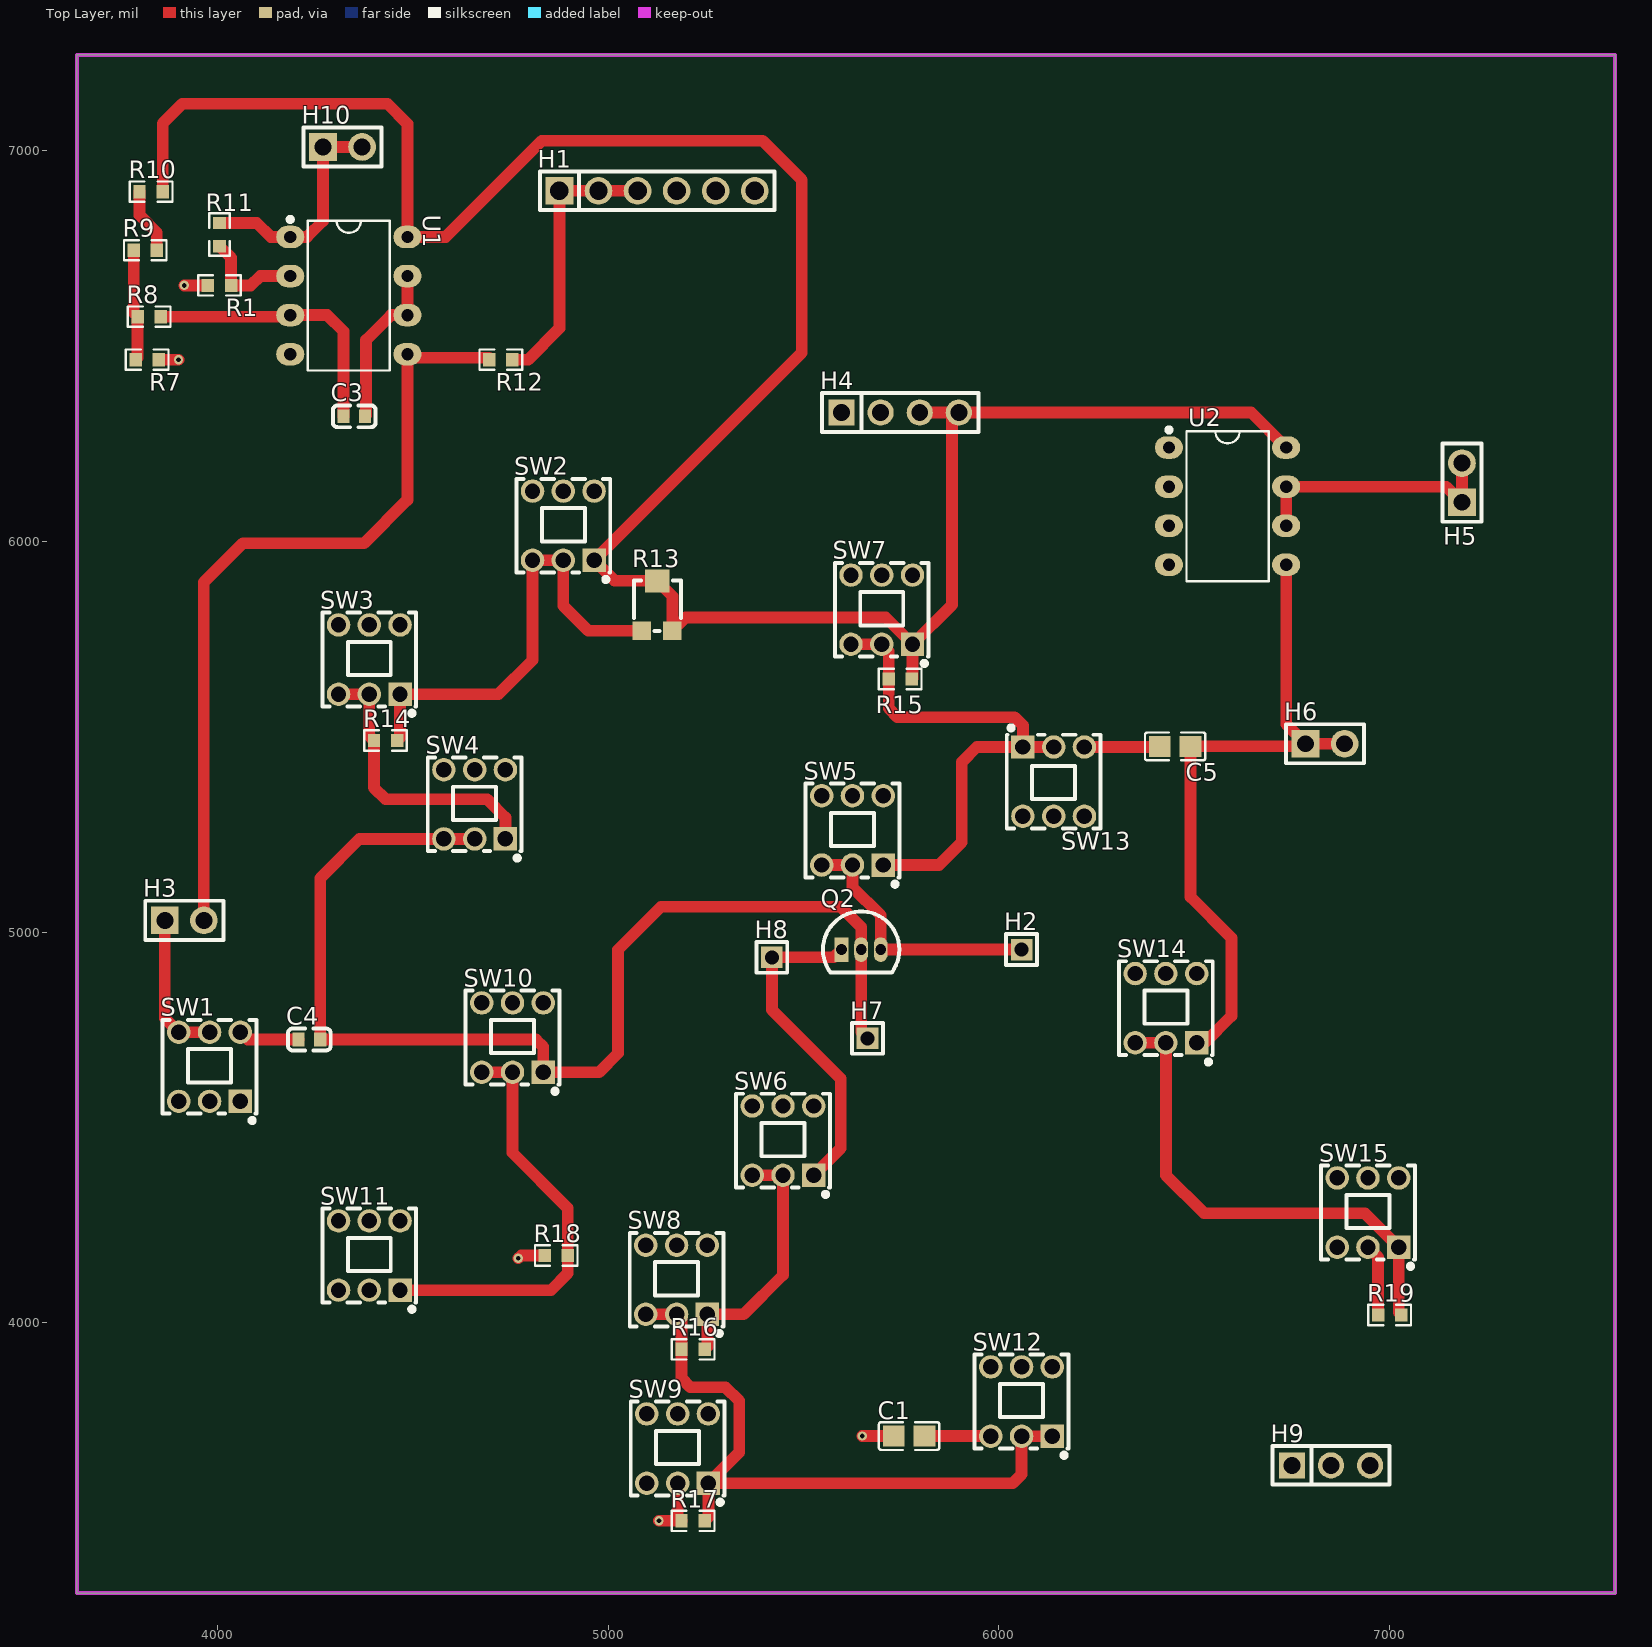
[diagram p0: Top Layer view]
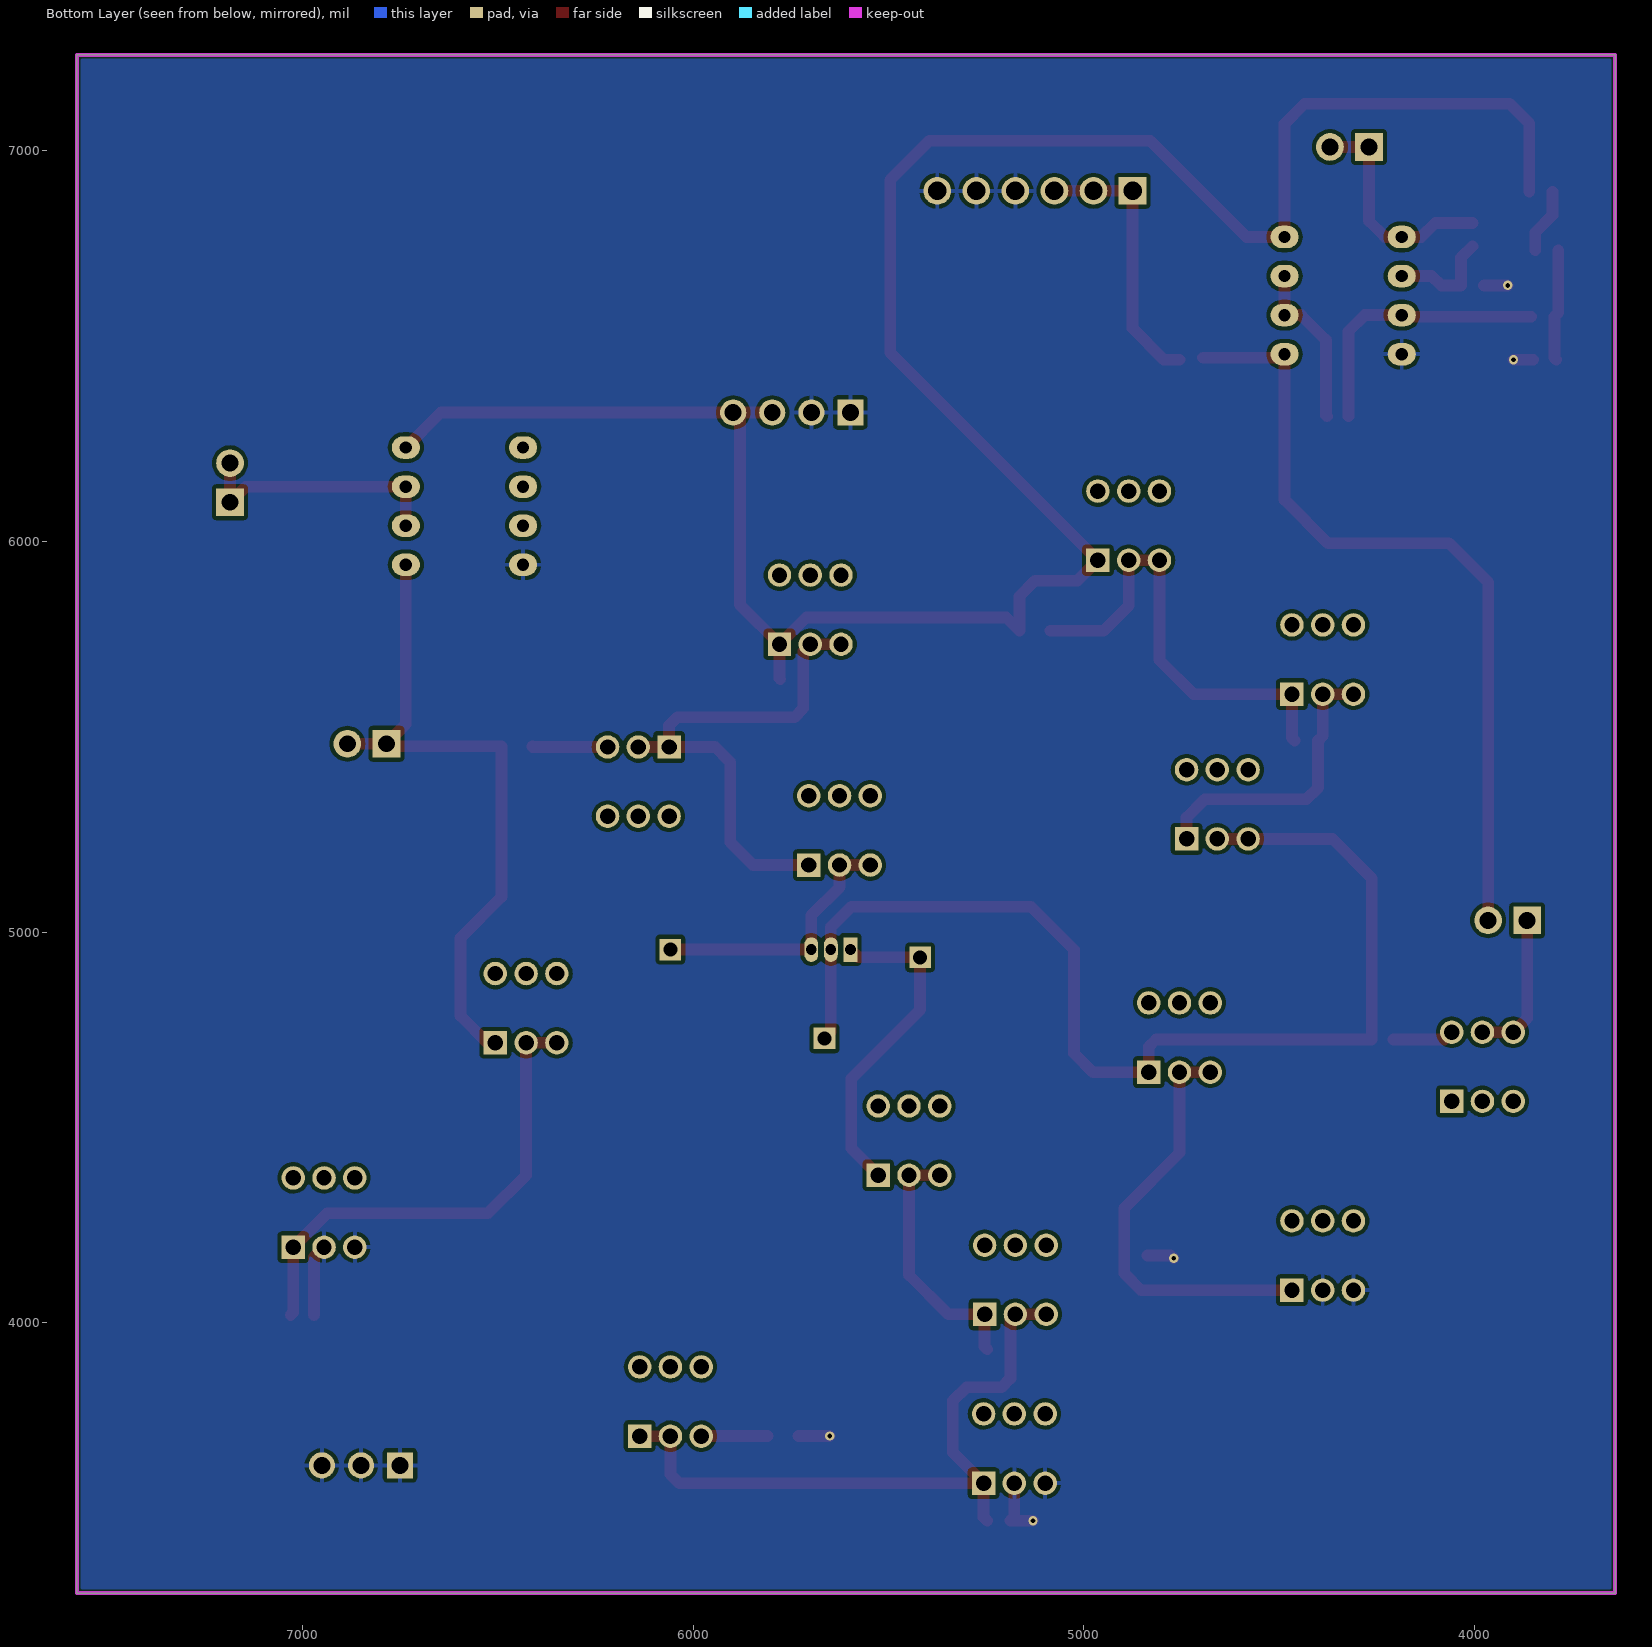
[diagram p1: Bottom Layer view, seen from below]
# Altium PCB MISC52134.pcbdoc
Units mil, origin at the board's own origin, x right, y up, seen from the top; angles counter-clockwise.
Board outline 3937.01 x 3937.01 mil, 2 copper layers (Top Layer, Bottom Layer), stack 62.206 mil thick; 46 components, 26 nets, 170 pads, 5 vias.

## Layer stack, top to bottom
Top Solder Mask Layer: solder mask 0.394, Dk 3.3
Top Layer: signal copper 1.379
Dielectric1: surface 59.449, FR4, Dk 4.5
Bottom Layer: signal copper 1.378
Bottom Solder Mask Layer: solder mask 0.394, Dk 3.3

## Board outline
3640,7245 3640,3307.99 7577.01,3307.99 7577.01,7245

## Design rules (kind name [scope] priority, off if disabled: settings)
BoardOutlineClearance copperThickness2oz_1 [All] p2 off: genericclearance=7.99 ignorepadtopadclearanceinfootprint=FALSE except(0: Arc-SplitContinuation Track-SplitContinuation SMDPad-SplitContinuation THPad-SplitContinuation Via-SplitContinuation Fill-SplitContinuation Region-SplitContinuation Poly-SplitContinuation Text-SplitContinuation Hole-SplitContinuation; 5.98: Arc-CutoutEdge SMDPad-CutoutEdge THPad-CutoutEdge Via-CutoutEdge Fill-CutoutEdge Region-CutoutEdge Text-CutoutEdge; 6.93: Hole-OutlineEdge Hole-CutoutEdge; 10: Poly-OutlineEdge Poly-CutoutEdge; 11.81: Arc-OutlineEdge Track-OutlineEdge SMDPad-OutlineEdge THPad-OutlineEdge Via-OutlineEdge Fill-OutlineEdge Region-OutlineEdge Text-OutlineEdge Track-CutoutEdge)
BoardOutlineClearance copperThickness1oz_1 [All] p4: genericclearance=4.02 ignorepadtopadclearanceinfootprint=FALSE except(0: Arc-SplitContinuation Track-SplitContinuation SMDPad-SplitContinuation THPad-SplitContinuation Via-SplitContinuation Fill-SplitContinuation Region-SplitContinuation Poly-SplitContinuation Text-SplitContinuation Hole-SplitContinuation; 6: SMDPad-CutoutEdge THPad-CutoutEdge Via-CutoutEdge Fill-CutoutEdge Region-CutoutEdge Text-CutoutEdge; 6.93: Hole-OutlineEdge Hole-CutoutEdge; 10: Poly-OutlineEdge Poly-CutoutEdge; 11.8: Arc-OutlineEdge Track-OutlineEdge SMDPad-OutlineEdge THPad-OutlineEdge Via-OutlineEdge Fill-OutlineEdge Region-OutlineEdge Text-OutlineEdge; 11.81: Arc-CutoutEdge Track-CutoutEdge)
Clearance copperThickness2oz [All] p1 off: gap=7.99 ignorepadtopadclearanceinfootprint=FALSE except(5.98: SMDPad-Track SMDPad-SMDPad THPad-Track SMDPad-THPad THPad-THPad Track-Via SMDPad-Via THPad-Via Via-Via Fill-Track Region-Track Fill-SMDPad Region-SMDPad Fill-THPad Region-THPad Fill-Via Region-Via Fill-Fill Fill-Region Region-Region Arc-Track Arc-SMDPad Arc-THPad Arc-Via Fill-Arc Region-Arc Arc-Arc Text-Track SMDPad-Text Text-THPad Text-Via Fill-Text Region-Text Arc-Text Text-Text; 6.93: Hole-Track Hole-SMDPad Hole-THPad Hole-Via Fill-Hole Region-Hole Hole-Arc Hole-Text; 10: Poly-Track Poly-SMDPad Poly-THPad Poly-Via Poly-Fill Poly-Region Poly-Poly Poly-Arc Poly-Text Poly-Hole)
Clearance copperThickness1oz [All] p3: gap=4.02 ignorepadtopadclearanceinfootprint=FALSE except(5.98: SMDPad-Track SMDPad-SMDPad THPad-Track SMDPad-THPad THPad-THPad Track-Via SMDPad-Via THPad-Via Via-Via Fill-Track Region-Track Fill-SMDPad Region-SMDPad Fill-THPad Region-THPad Fill-Via Region-Via Fill-Fill Fill-Region Region-Region; 6: Arc-Track Arc-SMDPad Arc-THPad Arc-Via Fill-Arc Region-Arc Arc-Arc Text-Track SMDPad-Text Text-THPad Text-Via Fill-Text Region-Text Arc-Text Text-Text; 6.93: Hole-Track Hole-SMDPad Hole-THPad Hole-Via Fill-Hole Region-Hole Hole-Arc Hole-Text; 10: Poly-Track Poly-SMDPad Poly-THPad Poly-Via Poly-Fill Poly-Region Poly-Poly Poly-Arc Poly-Text Poly-Hole)
Creepage creepage [All] p1: checkdistance=0 ignoreinternallayers=TRUE applytopolygonpour=TRUE
DiffPairsRouting differentialPair [All] p1: maxlimit=6 minlimit=6 mostfreqgap=6 toplayer_minwidth=5 toplayer_prefwidth=10 toplayer_maxwidth=100 toplayer_mingap=6 toplayer_prefgap=6 toplayer_maxgap=6 bottomlayer_minwidth=5 bottomlayer_prefwidth=10 bottomlayer_maxwidth=100 bottomlayer_mingap=6 bottomlayer_prefgap=6 bottomlayer_maxgap=6 maxuncoupledlength=10
HoleToHoleClearance otherClearance [All] p1: gap=11.81 allowstackedmicrovias=TRUE
Length netLength [All] p1: minlimit=0 maxlimit=0
MatchedLengths netLengthTolerance [All] p1: tolerance=1000
PasteMaskExpansion pasteMaskExpansion [All] p1: expansion=0
PlaneConnect innerPlane [All] p1: planeconnectstyle=Relief reliefexpansion=20 reliefentries=4 reliefconductorwidth=10 reliefairgap=10
PolygonConnect copperRegion [(InNet('GND'))] p1: connectstyle=Relief reliefconductorwidth=10 reliefentries=4 polygonreliefangle="90 Angle" airgapwidth=10 via.connectstyle=Relief via.reliefconductorwidth=10 via.reliefentries=4 via.polygonreliefangle="90 Angle" via.airgapwidth=10
RoutingVias viaSize [All] p1: holewidth=12.01 width=24.02 viastyle="Through Hole" minholewidth=11.81 minwidth=19.68 maxholewidth=248.03 maxwidth=393.7
SolderMaskExpansion solderMaskExpansion [IsVia] p1: expansion=-1000 istentingtop=TRUE
SolderMaskExpansion solderMaskExpansion [All] p2: expansion=2 istentingtop=FALSE
Width copperThickness2oz_2 [All] p1 off: maxlimit=100 minlimit=8 preferedwidth=10
Width copperThickness1oz_2 [All] p2: maxlimit=100 minlimit=5 preferedwidth=10

## Components (designator, comment, footprint, x,y, rotation, side; value= is the part's Value field where it differs from the comment)
C1 "100uF" C0805 5770,3710 r0 top
C3 "0.47uF" C0603 4350,6320 r0 top
C4 "10uF" C0603 4235,4725 r0 top
C5 "10uF" C0805 6450.98,5475.15 r180 top
H1 "" HDR-TH_6P-P2.54-V-M-1 5125,6897.06 r0 top
H2 "" HDR-TH_1P-V-M_XKB_X4611WV-01I-C28D40 6057.89,4955.13 r0 top
H3 "" HDR-TH_2P-P2.54-V-M-1 3915,5030 r0 top
H4 "" HDR-TH_4P-P2.54-V-M 5747.25,6329.7 r0 top
H5 "" HDR-TH_2P-P2.54-V-M-1 7185,6150 r90 top
H6 "" HDR-TH_2P-P2.54-V-M-1 6834.77,5481.89 r0 top
H7 "" HDR-TH_1P-V-M_XKB_X4611WV-01I-C28D40 5663.51,4727.83 r0 top
H8 "" HDR-TH_1P-V-M_XKB_X4611WV-01I-C28D40 5418.84,4935.13 r0 top
H9 "" HDR-TH_3P-P2.54-V-M 6850,3635 r0 top
H10 "" HDR-TH_2P-P2.54-V-M-1 4319.9,7009.39 r0 top
Q2 "2N2222A" TO-92-3_L4.9-W3.7-P1.27-L 5647.25,4955.13 r0 top
R1 "1kΩ" R0603 4005,6655 r180 top
R7 "1kΩ" R0603 3820,6465 r180 top
R8 "2kΩ" R0603 3825,6575 r0 top
R9 "100kΩ" R0603 3815,6745 r0 top
R10 "100kΩ" R0603 3830,6895 r0 top
R11 "20kΩ" R0603 4005,6785 r90 top
R12 "10KΩ" R0603 4725,6465 r180 top
R13 "100kΩ" RES-ADJ-SMD_JER33X-1-14 5125,5835 r0 top
R14 "39kΩ" R0603 4430,5490 r0 top
R15 "24kΩ" R0603 5747.25,5647.42 r0 top
R16 "100Ω" R0603 5217.25,3932.06 r0 top
R17 "1kΩ" R0603 5217.25,3493.05 r0 top
R18 "20KΩ" R0603 4866.92,4172.06 r0 top
R19 "2.4KΩ" R0603 7000,4020 r0 top
SW1 "5.8 ZSGT" SW-TH_5.8ZSGT 3979.58,4655.13 r0 top
SW2 "5.8 ZSGT" SW-TH_5.8ZSGT 4885,6040 r0 top
SW3 "5.8 ZSGT" SW-TH_5.8ZSGT 4388.4,5697.42 r0 top
SW4 "5.8 ZSGT" SW-TH_5.8ZSGT 4658.08,5326.89 r0 top
SW5 "5.8 ZSGT" SW-TH_5.8ZSGT 5625,5260 r0 top
SW6 "5.8 ZSGT" SW-TH_5.8ZSGT 5447.25,4466.08 r0 top
SW7 "5.8 ZSGT" SW-TH_5.8ZSGT 5700,5825 r0 top
SW8 "5.8 ZSGT" SW-TH_5.8ZSGT 5175,4110 r0 top
SW9 "5.8 ZSGT" SW-TH_5.8ZSGT 5177.56,3678.05 r0 top
SW10 "5.8 ZSGT" SW-TH_5.8ZSGT 4755,4730 r0 top
SW11 "5.8 ZSGT" SW-TH_5.8ZSGT 4388.4,4172.06 r0 top
SW12 "5.8 ZSGT" SW-TH_5.8ZSGT 6057.89,3798.37 r0 top
SW13 "5.8 ZSGT" SW-TH_5.8ZSGT 6140,5385 r180 top
SW14 "5.8 ZSGT" SW-TH_5.8ZSGT 6427.24,4805.13 r0 top
SW15 "5.8 ZSGT" SW-TH_5.8ZSGT 6944.45,4282.06 r0 top
U1 "LM358P" DIP-8_L9.4-W6.4-P2.54-LS9.1-BL 4336.02,6628.98 r270 top
U2 "LM358P" DIP-8_L9.4-W6.4-P2.54-LS9.1-BL 6585,6090 r270 top

## Footprints (in the part's own frame and the unit in brackets; to place one, negate y for a bottom-side part, rotate by r counter-clockwise, add the part's x,y. Pads: shape width x height; smd on the part's side, far side on the other; paste and mask are expansions set on the pad)
C0603 [mm]
  rect 0.8x0.9 smd: 1(-0.7,0) 2(0.7,0)
  silkscreen extent -1.39,-0.71 1.39,0.71
C0805 [mm]
  rect 1.41x1.35 smd paste-100 mask+0.051: 1(-1,0) 2(1,0)
  silkscreen extent -1.96,-0.9 1.96,0.9
DIP-8_L9.4-W6.4-P2.54-LS9.1-BL [mm]
  oval 1.46x1.825 hole 0.8: 1(-3.81,-3.81) 2(-1.27,-3.81) 3(1.27,-3.81) 4(3.81,-3.81) 5(3.81,3.81) 6(1.27,3.81) 7(-1.27,3.81) 8(-3.81,3.81)
  silkscreen extent -5.1,-3.96 4.87,2.67
HDR-TH_1P-V-M_XKB_X4611WV-01I-C28D40 [mm]
  rect 1.4x1.4 hole 0.9: 1(0,0)
  silkscreen extent -1,-1 1,1
HDR-TH_2P-P2.54-V-M-1 [mm]
  rect 1.8x1.8 hole 1.1: 1(-1.27,0)
  round 1.8 hole 1.1: 2(1.27,0)
  silkscreen extent -2.54,-1.27 2.54,1.27
HDR-TH_3P-P2.54-V-M [mm]
  rect 1.7x1.7 hole 1.1: 1(-2.54,0)
  round 1.7 hole 1.1: 2(0,0) 3(2.54,0)
  silkscreen extent -3.81,-1.25 3.81,1.25
HDR-TH_4P-P2.54-V-M [mm]
  rect 1.7x1.7 hole 1.1: 1(-3.81,0)
  round 1.7 hole 1.1: 2(-1.27,0) 3(1.27,0) 4(3.81,0)
  silkscreen extent -5.08,-1.27 5.08,1.27
HDR-TH_6P-P2.54-V-M-1 [mm]
  rect 1.8x1.8 hole 1.2: 1(-6.35,0)
  round 1.8 hole 1.2: 2(-3.81,0) 3(-1.27,0) 4(1.27,0) 5(3.81,0) 6(6.35,0)
  silkscreen extent -7.62,-1.25 7.62,1.25
R0603 [mil]
  rect 31.75x34.02 smd paste-3937.01 mask+2: 1(-29.66,0) 2(29.66,0)
  silkscreen extent -55,-26 55,26
RES-ADJ-SMD_JER33X-1-14 [mm]
  rect 1.2x1.2 smd paste+0 mask+0.05: 1(1,-1.625) 3(-1,-1.625)
  rect 1.6x1.5 smd paste+0 mask+0.05: 2(0,1.625)
  silkscreen extent -1.5,-1.65 1.55,1.65
SW-TH_5.8ZSGT [mm]
  rect 1.524x1.524 hole 1: 1(2,-2.25)
  round 1.524 hole 1: 2(0,-2.25) 3(-2,-2.25) 4(2,2.25) 5(0,2.25) 6(-2,2.25)
  silkscreen extent -3.05,-3.64 3.05,3.05
TO-92-3_L4.9-W3.7-P1.27-L [mm]
  rect 0.9x1.6 hole 0.7: 1(-1.27,0)
  oval 0.9x1.6 hole 0.7: 2(0,0) 3(1.27,0)
  silkscreen extent -2.48,-1.5 2.48,2.48

## Via types
v1: diameter 24.02, hole 12, Top Layer to Bottom Layer, 5 vias

## Nets (pads, with @x,y where several pads share a name; then routed paths per layer and width w, separated by ;. In a path a pad name is that pad's centre, name@x,y a point inside that pad or via, vN(x,y) a via of type N, cw(c..) or ccw(c..) an arc to the next point about the centre after c; other vN are vias at no path point)
$1N2: R7.2 R8.1 R9.1 | length 286.2
  Top Layer w30: R9.1 3785.34,6585 R8.1 3795.34,6470 R7.2
$1N3: R9.2 R10.1 | length 168.4
  Top Layer w30: R10.1 3800.34,6834.66 3844.66,6790.34 R9.2
$1N4: H4.3 H4.4 R10.2 R13.1 R13.2 R15.2 SW2.1 SW7.1 U1.8 U2.8 | length 6170.1
  Top Layer w30: R10.2 3859.66,7069.66 3910,7120 4435,7120 4486.02,7068.98 U1.8 4583.98,6778.98 4830,7025 5395,7025 5495,6925 5495,6482.68 SW2.1 5016.18,5898.98 R13.2 5164.37,5859.61 R13.1 5198.35,5805 5710.16,5805 SW7.1 ; R15.2 5778.74,5649.25 SW7.1 ; H4.3 H4.4 ; U2.8 6645.3,6329.7 H4.4 ; SW7.1 5880,5837.68 5880,6312.45 H4.4
$1N5: C3.2 U1.6 U1.7 | length 428.5
  Top Layer w30: C3.2 4380,6322.44 4380,6515 4443.98,6578.98 U1.6 U1.7
$1N6: C3.1 R8.2 U1.3 | length 704.1
  Top Layer w30: R8.2 4182.04,6575 U1.3 4281.02,6578.98 4322.44,6537.56 C3.1
$1N7: R1.1 R11.1 U1.2 | length 273.9
  Top Layer w30: R11.1 4034.66,6725.68 R1.1 4085,6655 4108.98,6678.98 U1.2
$1N9: H10.1 H10.2 R11.2 U1.1 | length 586.1
  Top Layer w30: R11.2 4100.34,6814.66 4136.02,6778.98 U1.1 4228.98,6778.98 4269.9,6819.9 H10.1 H10.2
$1N11: H3.2 R12.2 U1.5 | length 2059.2
  Top Layer w30: H3.2 3965,5895 4065,5995 4375,5995 4486.02,6106.02 U1.5 4495.34,6469.66 R12.2@4695,6469.66
$1N12: H1.1 H1.2 H1.3 R12.1 | length 705.5
  Top Layer w30: R12.1 4795,6465 4875,6545 H1.1 H1.2 H1.3
$1N13: H3.1 SW1.5 SW1.6 | length 379.9
  Top Layer w30: H3.1 3865,4779.56 SW1.6 SW1.5
$1N14: C4.1 SW1.4 | length 156.9
  Top Layer w30: SW1.4 4077.04,4725 C4.1
$1N17: H5.1 H5.2 U2.6 U2.7 | length 666.6
  Top Layer w30: U2.6 U2.7 7145,6140 H5.1 H5.2
$1N19: R13.3 R14.2 SW2.2 SW2.3 SW3.1 | length 1174.7
  Top Layer w30: R14.2 4467.14,5497.48 SW3.1 4718.83,5608.83 4806.26,5696.26 SW2.3 SW2.2 4885,5835 4948.98,5771.02 R13.3
$1N20: R14.1 SW3.2 SW3.3 SW4.1 | length 745.9
  Top Layer w30: SW3.3 SW3.2 4388.4,5501.94 R14.1 4400.34,5369.66 4430,5340 4690,5340 4736.82,5293.18 SW4.1
$1N21: C4.2 H7.1 Q2.2 SW4.2 SW4.3 SW10.1 | length 2951.1
  Top Layer w30: SW4.2 SW4.3 4363.31,5238.31 4262.56,5137.56 C4.2 4815,4725 4833.74,4706.26 SW10.1 4976.42,4641.42 5025,4690 5025,4955 5135,5065 5595,5065 5647.25,5012.75 Q2.2 5647.25,4744.09 H7.1
$1N22: H2.1 Q2.3 SW5.2 SW5.3 | length 685.6
  Top Layer w30: SW5.3 SW5.2 5625,5115 5697.25,5042.75 Q2.3 H2.1
$1N23: R16.2 SW6.2 SW6.3 SW8.1 | length 661.4
  Top Layer w30: R16.2 5253.74,3938.89 SW8.1 5346.42,4021.42 5447.25,4122.25 SW6.2 SW6.3
$1N24: H8.1 Q2.1 SW6.1 | length 845.9
  Top Layer w30: SW6.1 5595,4446.51 5595,4625 5418.84,4801.16 H8.1 5577.25,4935.13 Q2.1
$1N27: R15.1 SW5.1 SW7.2 SW7.3 SW13.1 SW13.2 | length 1348.5
  Top Layer w30: SW7.3 SW7.2 5717.59,5718.83 R15.1 5717.59,5572.41 5740,5550 6040,5550 6061.26,5528.74 SW13.1 ; SW5.1 5846.42,5171.42 5905,5230 5905,5435 5943.58,5473.58 SW13.1 ; SW13.2 SW13.1
$1N28: R16.1 R17.2 SW8.2 SW8.3 SW9.1 SW12.1 SW12.2 | length 1749.8
  Top Layer w30: SW8.3 SW8.2 5187.59,4008.83 R16.1 5187.59,3857.41 5210,3835 5300,3835 5335,3800 5335,3668.16 SW9.1 ; R17.2 5256.3,3502.44 SW9.1 ; SW12.1 SW12.2 6057.89,3612.35 6035,3589.46 SW9.1
$1N30: R18.2 SW10.2 SW10.3 SW11.1 | length 1099.5
  Top Layer w30: SW11.1 4853.48,4083.48 4896.58,4126.58 R18.2 4896.58,4293.42 4755,4435 SW10.2 SW10.3
$1N33: C1.2 SW12.3 | length 169.9
  Top Layer w30: C1.2 5978.94,3710 SW12.3
$1N34: C5.2 SW13.3 | length 193.5
  Top Layer w30: SW13.3 6410.05,5473.58 C5.2
$1N35: C5.1 H6.1 H6.2 SW14.1 U2.5 | length 1726.8
  Top Layer w30: SW14.1@6505.98,4716.55 6526.55,4716.55 6595,4785 6595,4985 6490.35,5089.65 C5.1 6778.03,5475.15 H6.1 ; U2.5 6735,5531.66 H6.1 ; H6.2 H6.1
$1N42: R19.2 SW14.2 SW14.3 SW15.1 | length 1266
  Top Layer w30: SW14.3@6348.5,4716.55 6427.24,4716.55 6427.24,4377.76 6525,4280 6936.67,4280 SW15.1 7023.19,4026.47 R19.2
GND: C1.1 H1.4 H1.5 H1.6 H4.1 H4.2 H9.1 H9.2 H9.3 R1.2 R7.1 R17.1 R18.1 R19.1 SW9.2 SW9.3 SW11.2 SW11.3 SW15.2 SW15.3 U1.4 U2.4 | length 603.9
  Top Layer w30: R7.1 v1(3900,6465) ; v1(3915,6655) R1.2 ; v1(4770,4165) 4777.06,4172.06 R18.1 ; v1(5130,3493.05) R17.1 5177.56,3503.07 SW9.2 ; v1(5650,3710) C1.1 ; SW15.2 6970.34,4167.59 R19.1
pads on no net: SW1.1 SW1.2 SW1.3 SW2.4 SW2.5 SW2.6 SW3.4 SW3.5 SW3.6 SW4.4 SW4.5 SW4.6 SW5.4 SW5.5 SW5.6 SW6.4 SW6.5 SW6.6 SW7.4 SW7.5 SW7.6 SW8.4 SW8.5 SW8.6 SW9.4 SW9.5 SW9.6 SW10.4 SW10.5 SW10.6 SW11.4 SW11.5 SW11.6 SW12.4 SW12.5 SW12.6 SW13.4 SW13.5 SW13.6 SW14.4 SW14.5 SW14.6 SW15.4 SW15.5 SW15.6 U2.1 U2.2 U2.3

## Polygon pours and split planes (outlines as drawn)
GND on Bottom Layer (solid, remove dead copper, pour order 0): 3000,7635 3000,3000 7905,3000 7905,7635

## Keep-outs
Board Outline Layer:
  the board outline again, w10